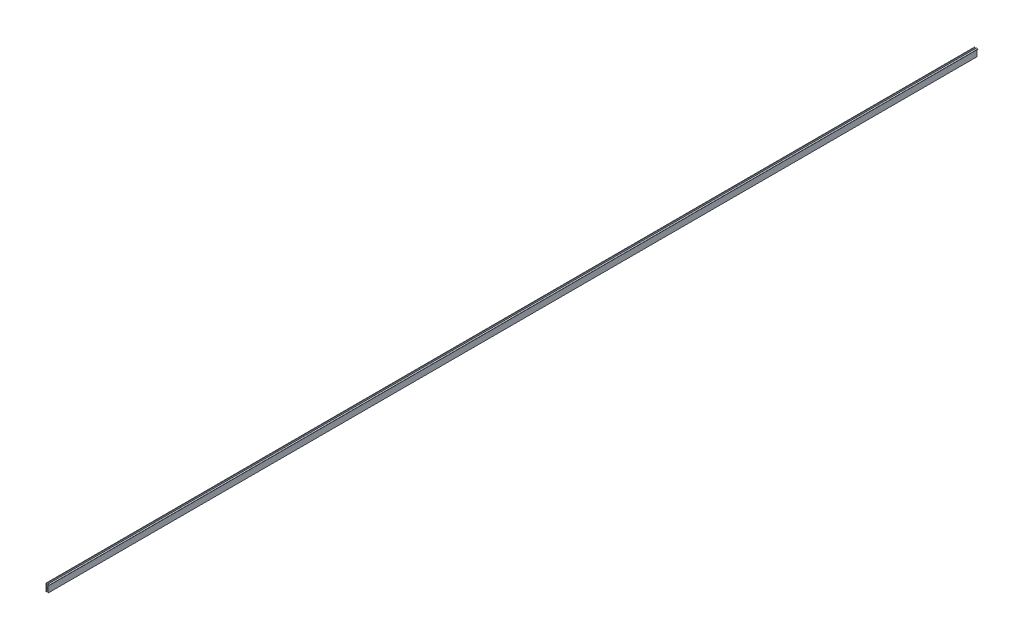
SolidWorks part; units mm, degrees
ref_plane "前视基准面" through (0, 0, 0) normal (0, 0, 1) x (1, 0, 0)
ref_plane "上视基准面" through (0, 0, 0) normal (0, 1, 0) x (1, 0, 0)
ref_plane "右视基准面" through (0, 0, 0) normal (1, 0, 0) x (0, 0, -1)
sketch "草图1" plane through (0, 0, 0) normal (0, 0, 1) x (1, 0, 0)
  line L0 (7.2551, 0) -> (3.2551, 0)
  line L1 (3.2551, 0) -> (3.2551, -8.6862)
  line L2 (3.2551, -8.6862) -> (-0.2449, -8.6862)
  line L3 (-0.2449, -8.6862) -> (-0.2449, 0)
  line L4 (-0.2449, 0) -> (-1.2449, 0)
  line L5 (-1.2449, 0) -> (-1.2449, -18.4)
  line L6 (-1.2449, -18.4) -> (-0.2449, -18.4)
  line L7 (-0.2449, -18.4) -> (-0.2449, -10.6862)
  line L8 (-0.2449, -10.6862) -> (3.2551, -10.6862)
  line L9 (3.2551, -10.6862) -> (3.2551, -18.6862)
  line L10 (3.2551, -18.6862) -> (4.2551, -18.6862)
  line L11 (4.2551, -18.6862) -> (4.2551, -0.7862)
  line L12 (4.2551, -0.7862) -> (7.2551, -0.7862)
  line L13 (7.2551, -0.7862) -> (7.2551, 0)
  dimension "D1" = 18.4
  dimension "D2" = 8.5
  dimension "D3" = 5.5
  dimension "D4" = 17.9
  dimension "D5" = 1
  dimension "D6" = 1
  dimension "D7" = 1
  dimension "D8" = 1
  dimension "D9" = 8
  dimension "D10" = 2
extrude "凸台-拉伸1" add sketch "草图1" along normal blind 2317
equation "\"A\" =1195"
equation "\"B\" =1155"
equation "\"CH\" = 2300"
equation "\"OP\" =750"
equation "\"OPH\" = 2100"
equation "\"QB\" = 50"
equation "\"DK\" = 40"
equation "\"WCOP\" =0"
equation "\"HCOP\" =4"
equation "\"FJ\" = 2"
equation "\"DH\" = 16"
equation "\"LG\" = 1"
equation "\"DD\" = 2"
equation "\"C\" =545"
equation "\"PX\" =-75"
equation "\"LZ\" = 350"
equation "\"LJ\" = 1158"
equation "\"LLK\" = 310"
equation "\"FS\" = 0"
equation "\"后玻璃框（纵）\"= \"CH\" + \"DH\" + 1"
equation "\"D1@凸台-拉伸1\"=\"后玻璃框（纵）\""
